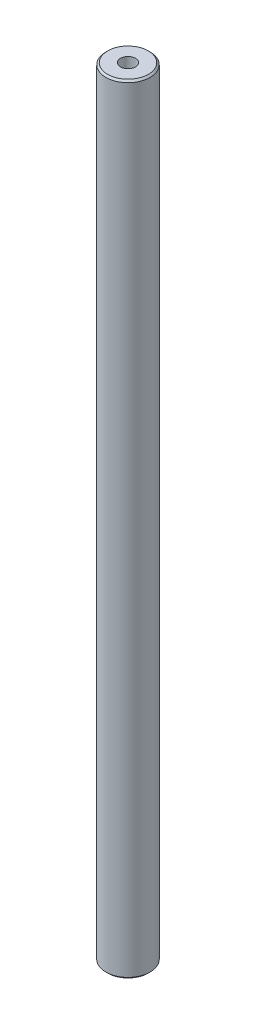
SolidWorks part; units mm, degrees
ref_plane "Front" through (0, 0, 0) normal (0, 0, 1) x (1, 0, 0)
ref_plane "Top" through (0, 0, 0) normal (0, 1, 0) x (1, 0, 0)
ref_plane "Right" through (0, 0, 0) normal (1, 0, 0) x (0, 0, -1)
sketch "草图1" plane through (0, 0, 0) normal (0, 1, 0) x (1, 0, 0)
  circle A0 centre (0, 0) radius 12.5
  dimension "D1" = 25
extrude "凸台-拉伸1" add sketch "草图1" along normal blind 440
chamfer "倒角1" distance 1 angle 45 2 edges at (0, 0, 12.5) (0, 440, 12.5)
hole_wizard "M10 螺纹孔1" positions "草图3" profile "草图2" tap size "M10" standard "Iso"
sketch "草图3" plane through (0, 440, 0) normal (0, 1, 0) x (1, 0, 0)
  point P0 (0, 0)
sketch "草图2" plane through (0, 440, 0) normal (1, 0, 0) x (0, 0, 1)
  line L0 (0, 0) -> (0, 29.0537)
  line L1 (0, 29.0537) -> (4.25, 26.5)
  line L2 (4.25, 26.5) -> (4.25, 0)
  line L5 (4.25, 0) -> (0, 0)
  line L10 (0, 29.0537) -> (-4.25, 26.5) construction
  line L11 (0, -6.35) -> (0, 107.95) construction
  dimension "螺纹孔钻头直径" = 8.5
  dimension "螺纹孔钻头深度" = 26.5
  dimension "导头角度" = 118
cosmetic thread "孔螺蚊线1" parameters "D1"=22, "D2"=10
